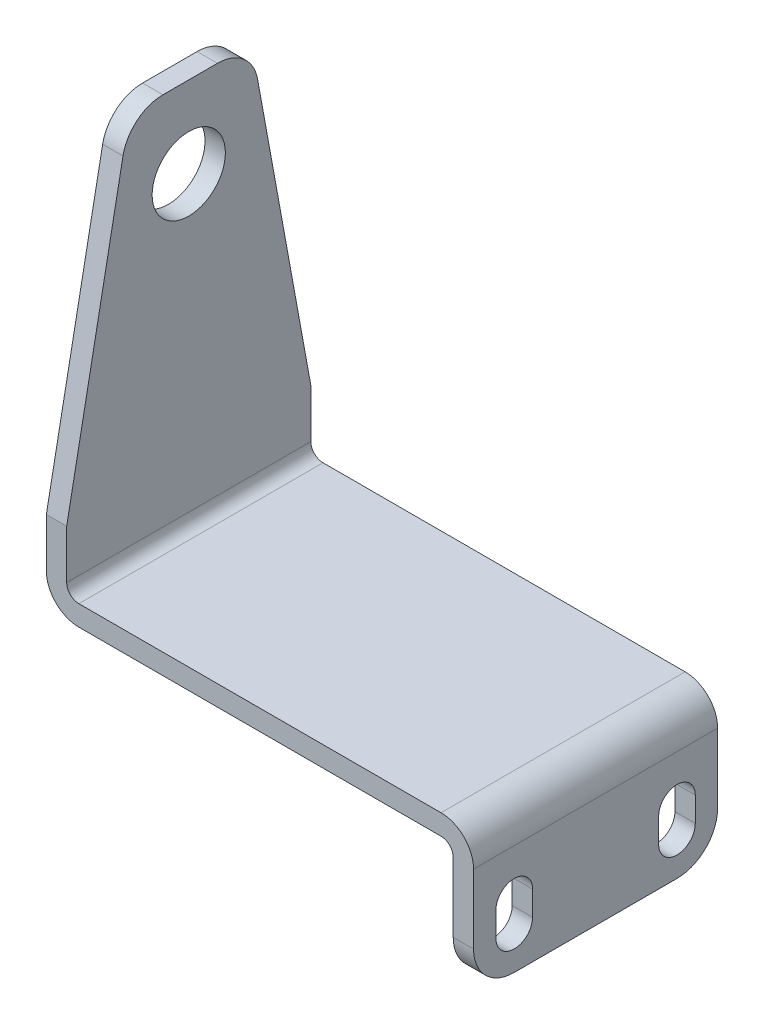
SolidWorks part; units mm, degrees
material "1023 碳钢板 (SS)"
ref_plane "Front Plane" through (0, 0, 0) normal (0, 0, 1) x (1, 0, 0)
ref_plane "Top Plane" through (0, 0, 0) normal (0, 1, 0) x (1, 0, 0)
ref_plane "Right Plane" through (0, 0, 0) normal (1, 0, 0) x (0, 0, -1)
sketch "Sketch1" plane through (0, 0, 0) normal (1, 0, 0) x (0, 0, -1)
  line L0 (0, -80) -> (-14.6006, 0)
  line L1 (-14.6006, 0) -> (-44.6006, 0)
  line L2 (-44.6006, 0) -> (-60, -80)
  line L3 (-60, -80) -> (-60, -130)
  line L4 (-60, -130) -> (0, -130)
  line L5 (0, -130) -> (0, -80)
extrude "Boss-Extrude1" add sketch "Sketch1" against normal blind 5
sketch "Sketch2" plane through (0, 0, 0) normal (1, 0, 0) x (0, 0, -1)
  line L0 (0, -130) -> (-60, -130)
  line L1 (-60, -130) -> (-60, -95)
  line L2 (-60, -95) -> (0, -95)
  line L3 (0, -95) -> (0, -130)
extrude "Boss-Extrude2" add sketch "Sketch2" along normal blind 100
sketch "Sketch3" plane through (0, 0, 0) normal (0, 0, -1) x (-1, 0, 0)
  line L0 (-95, -100) -> (-95, -130)
  line L1 (-95, -130) -> (5, -130)
  line L2 (5, -130) -> (5, -100)
  line L3 (5, -100) -> (-95, -100)
extrude "Cut-Extrude1" cut sketch "Sketch3" against normal through all
sketch "Sketch4" plane through (95, 0, 0) normal (-1, 0, 0) x (0, 0, 1)
  line L0 (54.5, -120.5) -> (54.5, -114.5)
  line L1 (45.5, -114.5) -> (45.5, -120.5)
  arc A0 (45.5, -120.5) -> (54.5, -120.5) centre (50, -120.5) ccw
  arc A1 (54.5, -114.5) -> (45.5, -114.5) centre (50, -114.5) ccw
extrude "Cut-Extrude2" cut sketch "Sketch4" against normal through all
sketch "Sketch5" plane through (100, 0, 0) normal (1, 0, 0) x (0, 0, -1)
  line L0 (-14.5, -114.5) -> (-14.5, -120.5)
  line L1 (-5.5, -120.5) -> (-5.5, -114.5)
  arc A0 (-14.5, -120.5) -> (-5.5, -120.5) centre (-10, -120.5) ccw
  arc A1 (-5.5, -114.5) -> (-14.5, -114.5) centre (-10, -114.5) ccw
extrude "Cut-Extrude3" cut sketch "Sketch5" against normal through all
hole_wizard "Ø18.0 (18) Diameter Hole1" positions "Sketch7" profile "Sketch6" hole size "Ø18.0" standard "ANSI Metric"
sketch "Sketch7" plane through (-5, 0, 0) normal (-1, 0, 0) x (0, 0, 1)
  point P0 (30, -20)
sketch "Sketch6" plane through (-5, -20, 30) normal (0, 1, 0) x (0, 0, 1)
  line L0 (0, 0) -> (0, 105)
  line L1 (0, 105) -> (9, 105)
  line L2 (9, 105) -> (9, 0)
  line L5 (9, 0) -> (0, 0)
  line L11 (0, -6.35) -> (0, 107.95) construction
  dimension "通孔孔直径" = 18
  dimension "通孔孔深度" = 105
fillet "Fillet1" radius 3 2 edges at (0, -95, 30) (95, -100, 30)
fillet "Fillet2" radius 8 2 edges at (-5, -100, 30) (100, -95, 30)
fillet "Fillet3" radius 10 4 edges at (97.5, -130, 60) (97.5, -130, 0) (-2.5, 0, 14.6006) (-2.5, 0, 44.6006)
